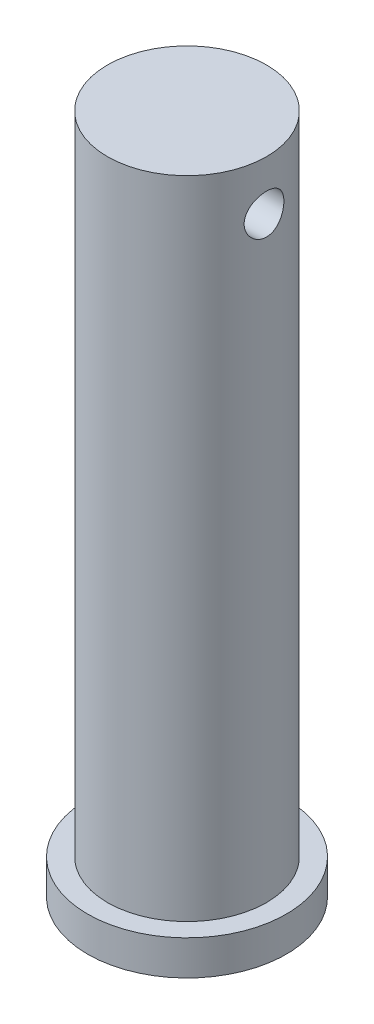
from build123d import *

# Parameters (mm, degrees)
SKETCH_2_R          = 2
CUT_EXTRUDE_1_DEPTH = 10


with BuildPart() as part:
    # 草图1 → 旋转1 (revolve)
    with BuildSketch(Plane.XY, mode=Mode.PRIVATE) as revolve_1_sk:
        Polygon((0, 34.25), (0, -34.25), (10, -34.25), (10, -30.75), (8, -30.75), (8, 34.25), align=None)
    revolve(revolve_1_sk.sketch.rotate(Axis((0, 34.25, 0), (0, -1, 0)), 90), axis=Axis((0, 34.25, 0), (0, -1, 0)))

    # 草图2 → 切除-拉伸1 (cut, symmetric)
    with BuildSketch(Plane(origin=(0, 0, 0), x_dir=(0, 0, -1), z_dir=(1, 0, 0))):
        with Locations((0, 29.25)):
            Circle(SKETCH_2_R)
    extrude(amount=CUT_EXTRUDE_1_DEPTH, both=True, mode=Mode.SUBTRACT)


solid = part.part
